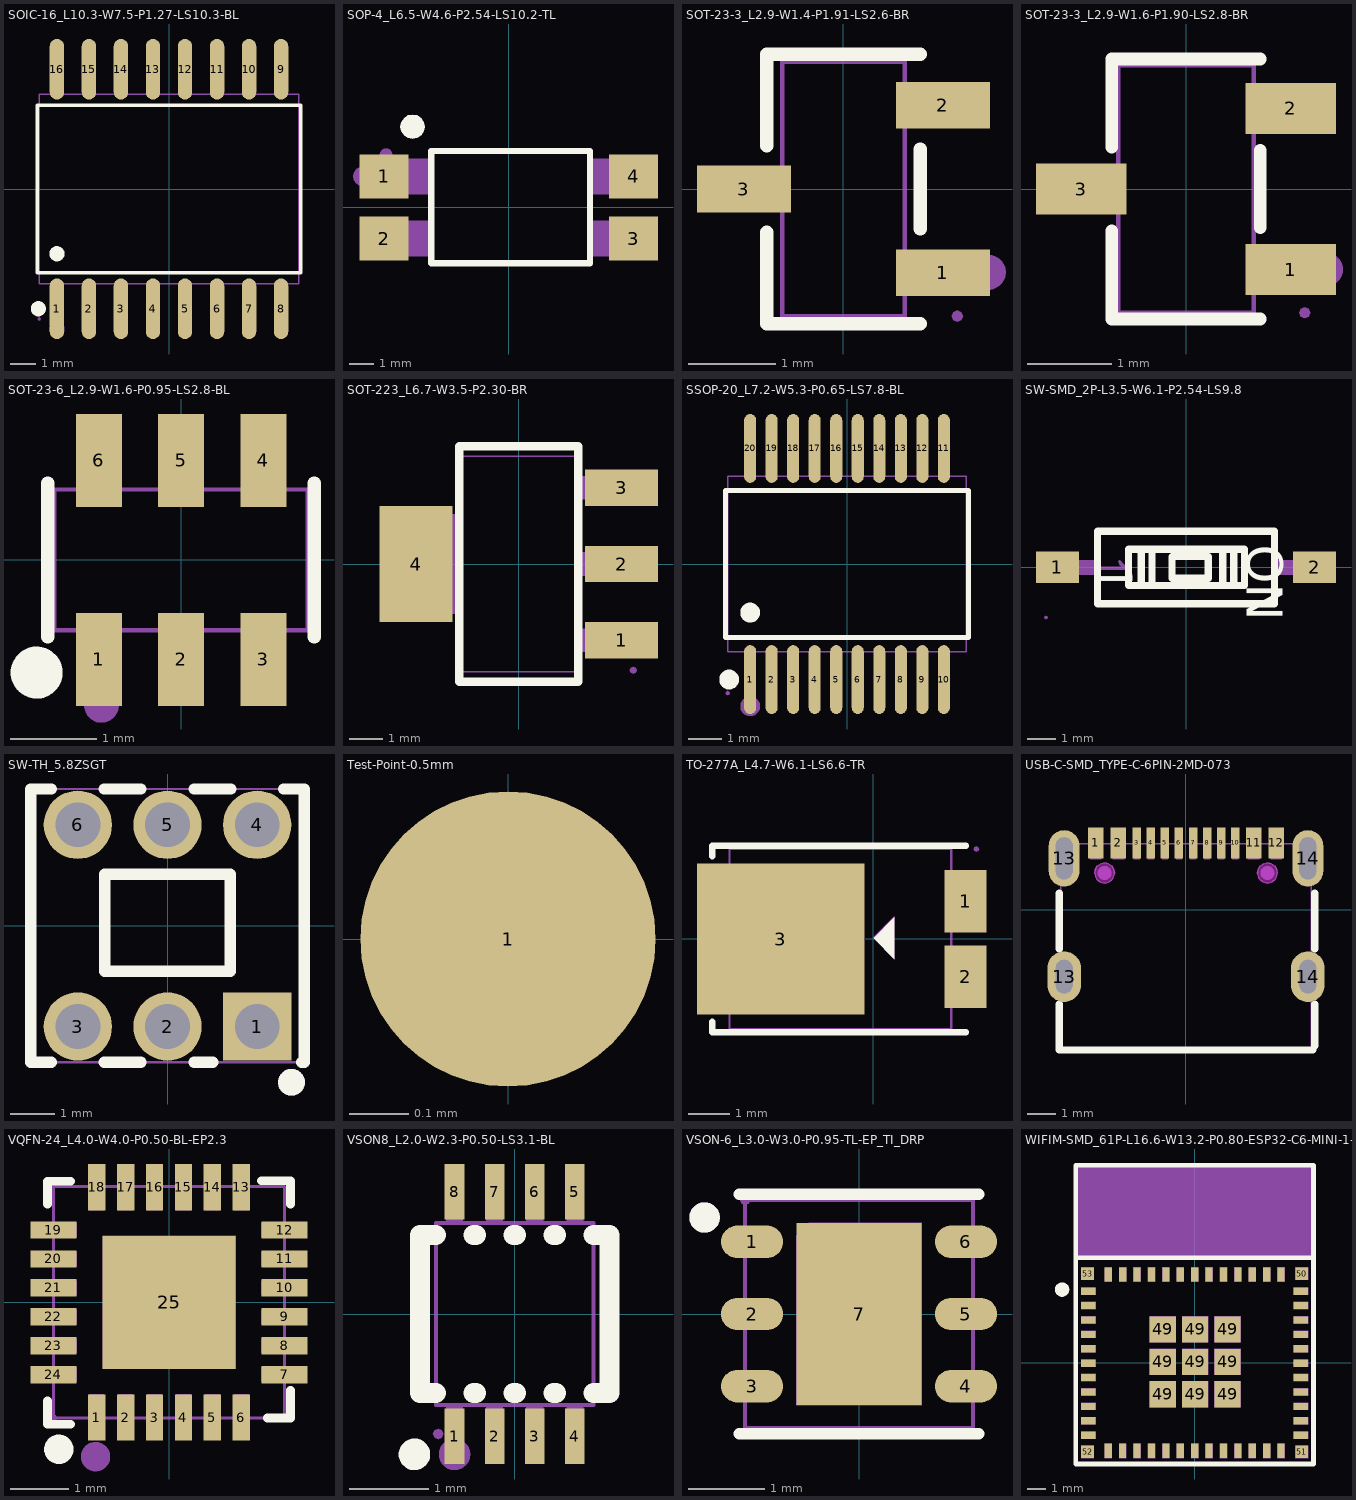
[diagram p0: the footprints below, top view; thin cyan lines are the x and y axes]
# Altium footprint library MISC84429-11.PcbLib: 64 footprints (part 4 of 4)
Each footprint in its own frame and in the unit in brackets; x right, y up, seen from the top. Pads: shape width x height; smd on the part's side, far side on the other; paste and mask are expansions set on the pad; w line width, h text height; cw(c..) or ccw(c..) is an arc to the next point about the centre after c.

## SOIC-16_L10.3-W7.5-P1.27-LS10.3-BL [mm]
pads (16):
  oval 0.574x2.401 smd: 1(-4.445,-4.75) 2(-3.175,-4.75) 3(-1.905,-4.75) 4(-0.635,-4.75) 5(0.635,-4.75) 6(1.905,-4.75) 7(3.175,-4.75) 8(4.445,-4.75) 9(4.445,4.75) 10(3.175,4.75) 11(1.905,4.75) 12(0.635,4.75) 13(-0.635,4.75) 14(-1.905,4.75) 15(-3.175,4.75) 16(-4.445,4.75)
Top Overlay:
  circle w0.3: c-5.184,-4.75 r0.15
  circle w0.3: c-4.445,-2.569 r0.15
  lines w0.152: -5.226,-3.321 5.226,-3.321 5.226,3.321 -5.226,3.321 -5.226,-3.321
Mechanical 6:
  circle w0.3: c-4.445,-5.563 r0.15
Mechanical 15:
  region: 4.24,4.338 4.24,3.74 4.65,3.74 4.65,4.338
  region: 4.24,5.162 4.24,4.327 4.65,4.327 4.65,5.162
  region: 2.97,4.338 2.97,3.74 3.38,3.74 3.38,4.338
  region: 2.97,5.162 2.97,4.327 3.38,4.327 3.38,5.162
  region: 1.7,4.338 1.7,3.74 2.11,3.74 2.11,4.338
  region: 1.7,5.162 1.7,4.327 2.11,4.327 2.11,5.162
  region: 0.43,4.338 0.43,3.74 0.84,3.74 0.84,4.338
  region: 0.43,5.162 0.43,4.327 0.84,4.327 0.84,5.162
  region: -0.84,4.338 -0.84,3.74 -0.43,3.74 -0.43,4.338
  region: -0.84,5.162 -0.84,4.327 -0.43,4.327 -0.43,5.162
  region: -2.11,4.338 -2.11,3.74 -1.7,3.74 -1.7,4.338
  region: -2.11,5.162 -2.11,4.327 -1.7,4.327 -1.7,5.162
  region: -3.38,4.338 -3.38,3.74 -2.97,3.74 -2.97,4.338
  region: -3.38,5.162 -3.38,4.327 -2.97,4.327 -2.97,5.162
  region: -4.65,4.338 -4.65,3.74 -4.24,3.74 -4.24,4.338
  region: -4.65,5.162 -4.65,4.327 -4.24,4.327 -4.24,5.162
  region: 4.24,-4.338 4.24,-3.74 4.65,-3.74 4.65,-4.338
  region: 4.24,-5.162 4.24,-4.327 4.65,-4.327 4.65,-5.162
  region: 2.97,-4.338 2.97,-3.74 3.38,-3.74 3.38,-4.338
  region: 2.97,-5.162 2.97,-4.327 3.38,-4.327 3.38,-5.162
  region: 1.7,-4.338 1.7,-3.74 2.11,-3.74 2.11,-4.338
  region: 1.7,-5.162 1.7,-4.327 2.11,-4.327 2.11,-5.162
  region: 0.43,-4.338 0.43,-3.74 0.84,-3.74 0.84,-4.338
  region: 0.43,-5.162 0.43,-4.327 0.84,-4.327 0.84,-5.162
  region: -0.84,-4.338 -0.84,-3.74 -0.43,-3.74 -0.43,-4.338
  region: -0.84,-5.162 -0.84,-4.327 -0.43,-4.327 -0.43,-5.162
  region: -2.11,-4.338 -2.11,-3.74 -1.7,-3.74 -1.7,-4.338
  region: -2.11,-5.162 -2.11,-4.327 -1.7,-4.327 -1.7,-5.162
  region: -3.38,-4.338 -3.38,-3.74 -2.97,-3.74 -2.97,-4.338
  region: -3.38,-5.162 -3.38,-4.327 -2.97,-4.327 -2.97,-5.162
  region: -4.65,-4.338 -4.65,-3.74 -4.24,-3.74 -4.24,-4.338
  region: -4.65,-5.162 -4.65,-4.327 -4.24,-4.327 -4.24,-5.162
  region: -5.085,-5.163 -5.104,-5.208 -5.15,-5.227 -5.196,-5.208 -5.215,-5.163 -5.196,-5.117 -5.15,-5.098 -5.104,-5.117
  lines w0.051: -5.15,-3.75 5.15,-3.75 5.15,3.75 -5.15,3.75 -5.15,-3.75

## SOP-4_L6.5-W4.6-P2.54-LS10.2-TL [mm]
pads (4):
  rect 2x1.8 smd: 1(-5.1,1.27) 2(-5.1,-1.27) 3(5.1,-1.27) 4(5.1,1.27)
Top Overlay:
  region: -4.433,3.302 -4.395,3.114 -4.288,2.953 -4.127,2.845 -3.937,2.807 -3.747,2.845 -3.586,2.953 -3.479,3.114 -3.441,3.303 -3.479,3.493 -3.586,3.654 -3.747,3.761 -3.937,3.799 -4.127,3.761 -4.288,3.654 -4.395,3.493 -4.433,3.305 -4.423,3.304
  lines w0.254: -3.175,-2.286 3.325,-2.286 3.325,2.314 -3.175,2.314 -3.175,-2.286
Mechanical 1:
  circle w0.4: c-5.969,1.27 r0.2
Mechanical 2:
  region: -4.764,2.163 -4.784,2.064 -4.84,1.98 -4.924,1.924 -5.023,1.904 -5.122,1.924 -5.206,1.98 -5.262,2.064 -5.282,2.163 -5.262,2.262 -5.206,2.346 -5.122,2.402 -5.023,2.422 -4.924,2.402 -4.84,2.346 -4.784,2.262
  region: -4.55,0.545 -5.15,0.545 -5.15,1.995 -4.55,1.995
  region: -3.24,0.545 -4.56,0.545 -4.56,1.995 -3.24,1.995
  region: -4.55,-1.995 -5.15,-1.995 -5.15,-0.545 -4.55,-0.545
  region: -3.24,-1.995 -4.56,-1.995 -4.56,-0.545 -3.24,-0.545
  region: 5.15,-1.995 4.55,-1.995 4.55,-0.545 5.15,-0.545
  region: 4.56,-1.995 3.24,-1.995 3.24,-0.545 4.56,-0.545
  region: 5.15,0.545 4.55,0.545 4.55,1.995 5.15,1.995
  region: 4.56,0.545 3.24,0.545 3.24,1.995 4.56,1.995
  lines w0.051: -3.25,-2.29 3.25,-2.29 3.25,2.29 -3.25,2.29 -3.25,-2.29

## SOT-23-3_L2.9-W1.4-P1.91-LS2.6-BR [mm]
pads (3):
  rect 1.07x0.532 smd: 1(1.135,-0.955) 2(1.135,0.955) 3(-1.135,0)
Top Overlay:
  lines w0.152: -0.876,-0.495 -0.876,-1.536 0.876,-1.536 ; -0.876,0.495 -0.876,1.536 0.876,1.536 ; 0.876,-0.455 0.876,0.455
Mechanical 1:
  circle w0.2: c1.651,-0.95 r0.1
Mechanical 2:
  region: 1.365,-1.45 1.346,-1.496 1.3,-1.515 1.254,-1.496 1.235,-1.45 1.254,-1.404 1.3,-1.385 1.346,-1.404
  region: -0.96,-0.212 -0.96,0.212 -0.69,0.212 -0.69,-0.212
  region: -1.3,-0.212 -1.3,0.212 -0.95,0.212 -0.95,-0.212
  region: 0.69,0.742 0.69,1.167 0.96,1.167 0.96,0.742
  region: 0.95,0.742 0.95,1.167 1.3,1.167 1.3,0.742
  region: 0.69,-1.167 0.69,-0.742 0.96,-0.742 0.96,-1.167
  region: 0.95,-1.167 0.95,-0.742 1.3,-0.742 1.3,-1.167
  lines w0.051: -0.7,-1.45 -0.7,1.45 0.7,1.45 0.7,-1.45 -0.7,-1.45

## SOT-23-3_L2.9-W1.6-P1.90-LS2.8-BR [mm]
pads (3):
  rect 1.07x0.6 smd: 1(1.235,-0.95) 2(1.235,0.95) 3(-1.235,0)
Top Overlay:
  lines w0.152: -0.876,-0.495 -0.876,-1.536 0.876,-1.536 ; -0.876,0.495 -0.876,1.536 0.876,1.536 ; 0.876,-0.455 0.876,0.455
Mechanical 1:
  circle w0.2: c1.651,-0.95 r0.1
Mechanical 2:
  region: 1.465,-1.46 1.446,-1.506 1.4,-1.525 1.354,-1.506 1.335,-1.46 1.354,-1.414 1.4,-1.395 1.446,-1.414
  region: 0.95,-1.15 0.95,-0.75 1.4,-0.75 1.4,-1.15
  region: 0.79,-1.15 0.79,-0.75 0.96,-0.75 0.96,-1.15
  region: 0.95,0.75 0.95,1.15 1.4,1.15 1.4,0.75
  region: 0.79,0.75 0.79,1.15 0.96,1.15 0.96,0.75
  region: -0.95,-0.2 -0.95,0.2 -1.4,0.2 -1.4,-0.2
  region: -0.96,-0.2 -0.96,0.2 -0.79,0.2 -0.79,-0.2
  lines w0.051: -0.8,-1.46 -0.8,1.46 0.8,1.46 0.8,-1.46 -0.8,-1.46

## SOT-23-6_L2.9-W1.6-P0.95-LS2.8-BL [mm]
pads (6):
  rect 0.532x1.072 smd: 1(-0.95,-1.149) 2(0,-1.149) 3(0.95,-1.149) 4(0.95,1.149) 5(0,1.149) 6(-0.95,1.149)
Top Overlay:
  circle w0.3: c-1.668,-1.301 r0.15
  lines w0.152: -1.539,-0.889 -1.539,0.889 ; 1.539,-0.889 1.539,0.889
Mechanical 1:
  circle w0.2: c-0.92,-1.68 r0.1
Mechanical 2:
  region: -1.398,-1.4 -1.417,-1.446 -1.463,-1.465 -1.509,-1.446 -1.528,-1.4 -1.509,-1.354 -1.463,-1.335 -1.417,-1.354
  region: -1.165,-0.925 -0.735,-0.925 -0.735,-1.4 -1.165,-1.4
  region: -1.165,-0.803 -0.735,-0.803 -0.735,-0.935 -1.165,-0.935
  region: -0.215,-0.925 0.215,-0.925 0.215,-1.4 -0.215,-1.4
  region: -0.215,-0.803 0.215,-0.803 0.215,-0.935 -0.215,-0.935
  region: 0.735,-0.925 1.165,-0.925 1.165,-1.4 0.735,-1.4
  region: 0.735,-0.803 1.165,-0.803 1.165,-0.935 0.735,-0.935
  region: 0.735,0.925 1.165,0.925 1.165,1.4 0.735,1.4
  region: 0.735,0.935 1.165,0.935 1.165,0.803 0.735,0.803
  region: -0.215,0.925 0.215,0.925 0.215,1.4 -0.215,1.4
  region: -0.215,0.935 0.215,0.935 0.215,0.803 -0.215,0.803
  region: -1.165,0.925 -0.735,0.925 -0.735,1.4 -1.165,1.4
  region: -1.165,0.935 -0.735,0.935 -0.735,0.803 -1.165,0.803
  lines w0.051: -1.463,-0.813 1.463,-0.813 1.463,0.813 -1.463,0.813 -1.463,-0.813

## SOT-223_L6.7-W3.5-P2.30-BR [mm]
pads (4):
  rect 2.2x1.1 smd: 1(3.099,-2.3) 2(3.099,0) 3(3.099,2.3)
  rect 2.2x3.5 smd: 4(-3.099,0)
Top Overlay:
  lines w0.254: -1.8,-3.55 1.8,-3.55 1.8,3.55 -1.8,3.55 -1.8,-3.55
Mechanical 1:
  circle w0.254: c3.683,-2.286 r0.127
Mechanical 2:
  region: 3.558,-3.2 3.527,-3.277 3.45,-3.308 3.373,-3.277 3.342,-3.2 3.373,-3.123 3.45,-3.092 3.527,-3.123
  region: 1.74,1.95 1.74,2.65 2.61,2.65 2.61,1.95
  region: 2.6,1.95 2.6,2.65 3.5,2.65 3.5,1.95
  region: 1.74,-0.35 1.74,0.35 2.61,0.35 2.61,-0.35
  region: 2.6,-0.35 2.6,0.35 3.5,0.35 3.5,-0.35
  region: 1.74,-2.65 1.74,-1.95 2.61,-1.95 2.61,-2.65
  region: 2.6,-2.65 2.6,-1.95 3.5,-1.95 3.5,-2.65
  region: -2.61,-1.5 -2.61,1.5 -1.74,1.5 -1.74,-1.5
  region: -3.5,-1.5 -3.5,1.5 -2.6,1.5 -2.6,-1.5
  lines w0.051: -1.75,-3.25 -1.75,3.25 1.75,3.25 1.75,-3.25 -1.75,-3.25

## SSOP-20_L7.2-W5.3-P0.65-LS7.8-BL [mm]
pads (20):
  oval 0.364x2.082 smd: 1(-2.925,-3.491) 2(-2.275,-3.491) 3(-1.625,-3.491) 4(-0.975,-3.491) 5(-0.325,-3.491) 6(0.325,-3.491) 7(0.975,-3.491) 8(1.625,-3.491) 9(2.275,-3.491) 10(2.925,-3.491) 11(2.925,3.491) 12(2.275,3.491) 13(1.625,3.491) 14(0.975,3.491) 15(0.325,3.491) 16(-0.325,3.491) 17(-0.975,3.491) 18(-1.625,3.491) 19(-2.275,3.491) 20(-2.925,3.491)
Top Overlay:
  circle w0.3: c-2.925,-1.469 r0.15
  circle w0.3: c-3.559,-3.491 r0.15
  lines w0.152: -3.676,-2.221 -3.676,2.221 3.676,2.221 3.676,-2.221 -3.676,-2.221
Mechanical 1:
  circle w0.3: c-2.925,-4.3 r0.15
Mechanical 2:
  drawing of 45 lines, arcs and shapes, not listed

## SW-SMD_2P-L3.5-W6.1-P2.54-LS9.8 [mm]
pads (2):
  rect 1.5x1.1 smd: 1(-4.5,0) 2(4.5,0)
Top Overlay:
  lines w0.254: -1.57,-0.635 -1.57,0.635 ; -1.189,-0.635 -1.189,0.635 ; 1.288,-0.635 1.288,0.635 ; 1.669,-0.635 1.669,0.635 ; -3.1,-1.27 -3.1,1.27 3.1,1.27 3.1,-1.27 -3.1,-1.27 ; -2.014,-0.635 2.05,-0.635 2.05,0.635 -2.014,0.635 -2.014,-0.635 ; -0.49,-0.381 0.78,-0.381 0.78,0.381 -0.49,0.381 -0.49,-0.381
  text "ON" at 2.134,0.787 h1.27
  text "1" at -3.13,0.19 h1.27
Mechanical 1:
  region: -2.315,0.26 -2.335,0.26 -2.375,0.22 -2.355,0.15 -2.315,0.08 -2.255,0.02 -3.075,0.02 -3.085,0.03 -3.105,0.03 -3.135,0 -3.135,-0.04 -3.125,-0.07 -3.095,-0.08 -2.105,-0.08 -2.09,-0.075 -2.08,-0.065 -2.07,-0.055 -2.065,-0.03 -2.075,-0.01 -2.095,0.02 -2.215,0.14 -2.275,0.24
Mechanical 2:
  region: -4.835,-1.75 -4.854,-1.796 -4.9,-1.815 -4.946,-1.796 -4.965,-1.75 -4.946,-1.704 -4.9,-1.685 -4.854,-1.704
  region: 3.09,-0.25 3.09,0.25 4.41,0.25 4.41,-0.25
  region: 4.4,-0.25 4.4,0.25 4.9,0.25 4.9,-0.25
  region: -4.41,-0.25 -4.41,0.25 -3.09,0.25 -3.09,-0.25
  region: -4.9,-0.25 -4.9,0.25 -4.4,0.25 -4.4,-0.25
  lines w0.051: -3.1,-1.27 -3.1,1.27 3.1,1.27 3.1,-1.27 -3.1,-1.27

## SW-TH_5.8ZSGT [mm]
pads (6):
  rect 1.524x1.524 hole 1: 1(2,-2.25)
  round 1.524 hole 1: 2(0,-2.25) 3(-2,-2.25) 4(2,2.25) 5(0,2.25) 6(-2,2.25)
Top Overlay:
  circle w0.3: c2.766,-3.493 r0.15
  lines w0.254: -2.591,-3.047 -3.048,-3.047 -3.048,3.047 -2.591,3.047 ; -1.409,-3.047 -0.591,-3.047 ; -1.409,3.047 -0.591,3.047 ; 0.591,-3.047 1.01,-3.047 ; 0.591,3.047 1.409,3.047 ; 2.591,3.047 3.048,3.047 ; 2.99,-3.047 3.048,-3.047 3.048,3.048 ; -1.397,-1.016 1.397,-1.016 1.397,1.143 -1.397,1.143 -1.397,-1.016
Mechanical 1:
  circle w0.3: c2.766,-3.493 r0.15
Mechanical 2:
  region: 3.113,-3.048 3.094,-3.094 3.048,-3.113 3.002,-3.094 2.983,-3.048 3.002,-3.002 3.048,-2.983 3.094,-3.002
  region: 2.408,2.25 2.377,2.094 2.288,1.962 2.156,1.873 2,1.842 1.844,1.873 1.712,1.962 1.623,2.094 1.592,2.25 1.623,2.406 1.712,2.538 1.844,2.627 2,2.658 2.156,2.627 2.288,2.538 2.377,2.406
  region: 0.408,2.25 0.377,2.094 0.288,1.962 0.156,1.873 0,1.842 -0.156,1.873 -0.288,1.962 -0.377,2.094 -0.408,2.25 -0.377,2.406 -0.288,2.538 -0.156,2.627 0,2.658 0.156,2.627 0.288,2.538 0.377,2.406
  region: -1.592,2.25 -1.623,2.094 -1.712,1.962 -1.844,1.873 -2,1.842 -2.156,1.873 -2.288,1.962 -2.377,2.094 -2.408,2.25 -2.377,2.406 -2.288,2.538 -2.156,2.627 -2,2.658 -1.844,2.627 -1.712,2.538 -1.623,2.406
  region: -1.592,-2.25 -1.623,-2.406 -1.712,-2.538 -1.844,-2.627 -2,-2.658 -2.156,-2.627 -2.288,-2.538 -2.377,-2.406 -2.408,-2.25 -2.377,-2.094 -2.288,-1.962 -2.156,-1.873 -2,-1.842 -1.844,-1.873 -1.712,-1.962 -1.623,-2.094
  region: 0.408,-2.25 0.377,-2.406 0.288,-2.538 0.156,-2.627 0,-2.658 -0.156,-2.627 -0.288,-2.538 -0.377,-2.406 -0.408,-2.25 -0.377,-2.094 -0.288,-1.962 -0.156,-1.873 0,-1.842 0.156,-1.873 0.288,-1.962 0.377,-2.094
  region: 2.408,-2.25 2.377,-2.406 2.288,-2.538 2.156,-2.627 2,-2.658 1.844,-2.627 1.712,-2.538 1.623,-2.406 1.592,-2.25 1.623,-2.094 1.712,-1.962 1.844,-1.873 2,-1.842 2.156,-1.873 2.288,-1.962 2.377,-2.094
  lines w0.051: -3.048,-3.048 3.048,-3.048 3.048,3.048 -3.048,3.048 -3.048,-3.048

## Test-Point-0.5mm [mm]
pads (1):
  round 0.5 smd: 1(0,0)

## TO-277A_L4.7-W6.1-LS6.6-TR [mm]
pads (3):
  rect 1x1.5 smd: 1(2.21,0.9) 2(2.21,-0.9)
  rect 4x3.6 smd: 3(-2.21,0)
Top Overlay:
  region: 0.01,0.02 0.51,0.52 0.51,-0.48
  lines w0.152: -3.844,-1.98 -3.844,-2.229 2.218,-2.229 ; -3.844,1.98 -3.844,2.229 2.218,2.229
Mechanical 1:
  region: 0,0.04 0.5,0.54 0.5,-0.46
Mechanical 2:
  region: 2.53,2.15 2.511,2.104 2.465,2.085 2.419,2.104 2.4,2.15 2.419,2.196 2.465,2.215 2.511,2.196
  region: -4.033,0.9 -3.538,0.9 -3.538,1.54 -0.238,1.54 -0.238,-1.52 -3.538,-1.52 -3.538,-0.9 -4.033,-0.899 -4.032,0
  region: 1.863,1.351 2.465,1.35 2.465,0.45 1.862,0.45 1.862,0.897
  region: 1.863,-0.451 2.465,-0.45 2.465,-1.35 1.862,-1.349 1.862,-0.913
  lines w0.051: -3.432,-2.15 -3.432,2.15 1.868,2.15 1.868,-2.15 -3.432,-2.15

## USB-C-SMD_TYPE-C-6PIN-2MD-073 [mm]
pads (16):
  rect 0.55x1.1 smd paste-100 mask+0.05: 1(-3.2,2.375) 2(-2.4,2.375) 11(2.4,2.375) 12(3.2,2.375)
  rect 0.3x1.1 smd paste-100 mask+0.05: 3(-1.75,2.375) 4(-1.25,2.375) 5(-0.75,2.375) 6(-0.25,2.375) 7(0.25,2.375) 8(0.75,2.375) 9(1.25,2.375) 10(1.75,2.375)
  oval 1.2x1.8 hole 0.6 slot 1.2 at 90 deg paste+0 mask-0.25: 13(-4.325,-2.375) 14(4.325,-2.375)
  oval 1.1x2 hole 0.6 slot 1.5 at 90 deg paste+0 mask-0.2: 13(-4.325,1.825) 14(4.325,1.825)
Top Overlay:
  lines w0.254: -4.5,-3.356 -4.5,-4.975 4.5,-4.975 ; -4.5,-1.394 -4.5,0.594 ; 4.572,-4.826 4.572,-3.353 ; 4.572,-1.397 4.572,0.597
Top Paste:
  drawing of 16 lines, arcs and shapes, not listed
Keep-Out Layer:
  circle w0.013: c-2.89,1.305 r0.35
  circle w0.013: c-2.89,1.305 r0.35
  circle w0.013: c2.89,1.305 r0.35
  circle w0.013: c2.89,1.305 r0.35
  board cut-out: -2.533,1.305 -2.56,1.168 -2.638,1.053 -2.753,0.975 -2.89,0.948 -3.026,0.975 -3.142,1.053 -3.22,1.168 -3.247,1.305 -3.22,1.441 -3.142,1.557 -3.026,1.635 -2.89,1.662 -2.753,1.635 -2.638,1.557 -2.56,1.441
  board cut-out: 3.247,1.305 3.22,1.168 3.142,1.053 3.027,0.975 2.89,0.948 2.754,0.975 2.638,1.053 2.56,1.168 2.533,1.305 2.56,1.441 2.638,1.557 2.754,1.635 2.89,1.662 3.027,1.635 3.142,1.557 3.22,1.441
  region: -2.533,1.305 -2.56,1.168 -2.638,1.053 -2.753,0.975 -2.89,0.948 -3.026,0.975 -3.142,1.053 -3.22,1.168 -3.247,1.305 -3.22,1.441 -3.142,1.557 -3.026,1.635 -2.89,1.662 -2.753,1.635 -2.638,1.557 -2.56,1.441
  region: 3.247,1.305 3.22,1.168 3.142,1.053 3.027,0.975 2.89,0.948 2.754,0.975 2.638,1.053 2.56,1.168 2.533,1.305 2.56,1.441 2.638,1.557 2.754,1.635 2.89,1.662 3.027,1.635 3.142,1.557 3.22,1.441
  region: -2.533,1.305 -2.56,1.168 -2.638,1.053 -2.753,0.975 -2.89,0.948 -3.026,0.975 -3.142,1.053 -3.22,1.168 -3.247,1.305 -3.22,1.441 -3.142,1.557 -3.026,1.635 -2.89,1.662 -2.753,1.635 -2.638,1.557 -2.56,1.441
  region: 3.247,1.305 3.22,1.168 3.142,1.053 3.027,0.975 2.89,0.948 2.754,0.975 2.638,1.053 2.56,1.168 2.533,1.305 2.56,1.441 2.638,1.557 2.754,1.635 2.89,1.662 3.027,1.635 3.142,1.557 3.22,1.441
  lines w0.005: -3.247,1.305 -3.22,1.441 -3.142,1.557 -3.026,1.635 -2.89,1.662 -2.753,1.635 -2.638,1.557 -2.56,1.441 -2.533,1.305 -2.56,1.168 -2.638,1.053 -2.753,0.975 -2.89,0.948 -3.026,0.975 -3.142,1.053 -3.22,1.168 -3.247,1.305 ; 2.533,1.305 2.56,1.441 2.638,1.557 2.754,1.635 2.89,1.662 3.027,1.635 3.142,1.557 3.22,1.441 3.247,1.305 3.22,1.168 3.142,1.053 3.027,0.975 2.89,0.948 2.754,0.975 2.638,1.053 2.56,1.168 2.533,1.305
Mechanical 1:
  circle w0.013: c-2.89,1.305 r0.35
  circle w0.013: c2.89,1.305 r0.35
  circle w0.25: c-2.89,1.305 r0.125
  circle w0.25: c2.89,1.305 r0.125
  lines w0.005: -3.247,1.305 -3.22,1.441 -3.142,1.557 -3.026,1.635 -2.89,1.662 -2.753,1.635 -2.638,1.557 -2.56,1.441 -2.533,1.305 -2.56,1.168 -2.638,1.053 -2.753,0.975 -2.89,0.948 -3.026,0.975 -3.142,1.053 -3.22,1.168 -3.247,1.305 ; 2.533,1.305 2.56,1.441 2.638,1.557 2.754,1.635 2.89,1.662 3.027,1.635 3.142,1.557 3.22,1.441 3.247,1.305 3.22,1.168 3.142,1.053 3.027,0.975 2.89,0.948 2.754,0.975 2.638,1.053 2.56,1.168 2.533,1.305
Mechanical 2:
  region: -4.385,2.649 -4.404,2.603 -4.45,2.584 -4.496,2.603 -4.515,2.649 -4.496,2.695 -4.45,2.714 -4.404,2.695
  region: -1.85,2.649 -1.65,2.649 -1.65,1.799 -1.85,1.799
  region: -0.85,2.649 -0.65,2.649 -0.65,1.799 -0.85,1.799
  region: -1.35,2.649 -1.15,2.649 -1.15,1.799 -1.35,1.799
  region: -0.35,2.649 -0.15,2.649 -0.15,1.799 -0.35,1.799
  region: 0.15,2.649 0.35,2.649 0.35,1.799 0.15,1.799
  region: 0.65,2.649 0.85,2.649 0.85,1.799 0.65,1.799
  region: 1.15,2.649 1.35,2.649 1.35,1.799 1.15,1.799
  region: 1.65,2.649 1.85,2.649 1.85,1.799 1.65,1.799
  region: -3.4,2.649 -3,2.649 -3,1.799 -3.4,1.799
  region: -2.6,2.649 -2.2,2.649 -2.2,1.799 -2.6,1.799
  region: 2.2,2.649 2.6,2.649 2.6,1.799 2.2,1.799
  region: 3,2.649 3.4,2.649 3.4,1.799 3,1.799
  region: -4.45,2.349 -4.2,2.349 -4.2,1.249 -4.45,1.249
  region: 4.2,2.349 4.45,2.349 4.45,1.249 4.2,1.249
  region: -4.45,-2.025 -4.2,-2.025 -4.2,-2.725 -4.45,-2.725
  region: 4.2,-2.025 4.45,-2.025 4.45,-2.725 4.2,-2.725
  lines w0.051: -4.45,-5.001 -4.45,2.349 4.45,2.349 4.45,-5.001 -4.45,-5.001

## VQFN-24_L4.0-W4.0-P0.50-BL-EP2.3 [mm]
pads (25):
  rect 0.3x0.8 smd paste-100 mask+0.051: 1(-1.25,-1.992) 2(-0.75,-1.991) 3(-0.25,-1.991) 4(0.25,-1.991) 5(0.75,-1.991) 6(1.25,-1.991) 13(1.25,1.992) 14(0.75,1.992) 15(0.25,1.992) 16(-0.25,1.992) 17(-0.75,1.992) 18(-1.25,1.992)
  rect 0.8x0.3 smd paste-100 mask+0.051: 7(1.998,-1.25) 8(1.998,-0.75) 9(1.998,-0.25) 10(1.998,0.25) 11(1.998,0.75) 12(1.998,1.25) 19(-1.998,1.25) 20(-1.998,0.75) 21(-1.998,0.25) 22(-1.998,-0.25) 23(-1.998,-0.75) 24(-1.998,-1.25)
  rect 2.3x2.3 smd paste-100 mask+0.051: 25(0.001,-0.001)
Top Overlay:
  circle w0.254: c-1.905,-2.54 r0.127
  lines w0.15: -2.1,1.696 -2.1,2.096 -1.7,2.096 ; -2.1,-1.7 -2.1,-2.104 -1.7,-2.104 ; 1.6,2.1 2.1,2.1 2.1,1.7 ; 1.7,-2 2.1,-2 2.1,-1.524
Top Paste:
  region: 1.4,1.592 1.4,2.392 1.1,2.392 1.1,1.592
  region: -1.4,2.392 -1.4,1.592 -1.1,1.592 -1.1,2.392
  region: 0.9,1.592 0.9,2.392 0.6,2.392 0.6,1.592
  region: 0.4,1.592 0.4,2.392 0.1,2.392 0.1,1.592
  region: -0.1,1.592 -0.1,2.392 -0.4,2.392 -0.4,1.592
  region: -0.9,2.392 -0.9,1.592 -0.6,1.592 -0.6,2.392
  region: 2.398,1.1 2.398,1.4 1.598,1.4 1.598,1.1
  region: -2.398,1.4 -2.398,1.1 -1.598,1.1 -1.598,1.4
  region: 0.95,-0.95 0.95,0.95 -0.95,0.95 -0.95,-0.95
  region: 1.598,0.9 1.598,0.6 2.398,0.6 2.398,0.9
  region: -2.398,0.9 -2.398,0.6 -1.598,0.6 -1.598,0.9
  region: -2.398,0.4 -2.398,0.1 -1.598,0.1 -1.598,0.4
  region: 1.598,0.4 1.598,0.1 2.398,0.1 2.398,0.4
  region: -2.398,-0.1 -2.398,-0.4 -1.598,-0.4 -1.598,-0.1
  region: 1.598,-0.1 1.598,-0.4 2.398,-0.4 2.398,-0.1
  region: -2.398,-0.6 -2.398,-0.9 -1.598,-0.9 -1.598,-0.6
  region: 1.598,-0.6 1.598,-0.9 2.398,-0.9 2.398,-0.6
  region: -2.398,-1.1 -2.398,-1.4 -1.598,-1.4 -1.598,-1.1
  region: 1.598,-1.1 1.598,-1.4 2.398,-1.4 2.398,-1.1
  region: 1.4,-2.391 1.4,-1.591 1.1,-1.591 1.1,-2.391
  region: 0.9,-2.391 0.9,-1.591 0.6,-1.591 0.6,-2.391
  region: -0.4,-1.591 -0.4,-2.391 -0.1,-2.391 -0.1,-1.591
  region: 0.4,-2.391 0.4,-1.591 0.1,-1.591 0.1,-2.391
  region: -0.9,-1.591 -0.9,-2.391 -0.6,-2.391 -0.6,-1.591
  region: -1.1,-2.392 -1.1,-1.592 -1.4,-1.592 -1.4,-2.392
Mechanical 1:
  circle w0.254: c-1.27,-2.667 r0.127
Mechanical 2:
  region: -1.935,-2 -1.954,-2.046 -2,-2.065 -2.046,-2.046 -2.065,-2 -2.046,-1.954 -2,-1.935 -1.954,-1.954
  region: -1.125,-1.992 -1.375,-1.992 -1.375,-1.592 -1.125,-1.592
  region: -0.625,-1.992 -0.875,-1.992 -0.875,-1.592 -0.625,-1.592
  region: -0.125,-1.992 -0.375,-1.992 -0.375,-1.592 -0.125,-1.592
  region: 0.375,-1.992 0.125,-1.992 0.125,-1.592 0.375,-1.592
  region: 0.875,-1.992 0.625,-1.992 0.625,-1.592 0.875,-1.592
  region: 1.375,-1.992 1.125,-1.992 1.125,-1.592 1.375,-1.592
  region: 1.598,-1.375 1.598,-1.125 1.998,-1.125 1.998,-1.375
  region: 1.598,-0.875 1.598,-0.625 1.998,-0.625 1.998,-0.875
  region: 1.598,-0.375 1.598,-0.125 1.998,-0.125 1.998,-0.375
  region: 1.598,0.125 1.598,0.375 1.998,0.375 1.998,0.125
  region: 1.598,0.625 1.598,0.875 1.998,0.875 1.998,0.625
  region: 1.598,1.125 1.598,1.375 1.998,1.375 1.998,1.125
  region: 1.125,1.992 1.375,1.992 1.375,1.592 1.125,1.592
  region: 0.625,1.992 0.875,1.992 0.875,1.592 0.625,1.592
  region: 0.125,1.992 0.375,1.992 0.375,1.592 0.125,1.592
  region: -0.375,1.992 -0.125,1.992 -0.125,1.592 -0.375,1.592
  region: -0.875,1.992 -0.625,1.992 -0.625,1.592 -0.875,1.592
  region: -1.375,1.992 -1.125,1.992 -1.125,1.592 -1.375,1.592
  region: -1.598,1.375 -1.598,1.125 -1.998,1.125 -1.998,1.375
  region: -1.598,0.875 -1.598,0.625 -1.998,0.625 -1.998,0.875
  region: -1.598,0.375 -1.598,0.125 -1.998,0.125 -1.998,0.375
  region: -1.598,-0.125 -1.598,-0.375 -1.998,-0.375 -1.998,-0.125
  region: -1.598,-0.625 -1.598,-0.875 -1.998,-0.875 -1.998,-0.625
  region: -1.598,-1.125 -1.598,-1.375 -1.998,-1.375 -1.998,-1.125
  region: -1.149,-1.151 -1.149,1.149 1.151,1.149 1.151,-1.151
  lines w0.051: -2,-2 2,-2 2,2 -2,2 -2,-2

## VSON8_L2.0-W2.3-P0.50-LS3.1-BL [mm]
pads (8):
  rect 0.25x0.7 smd: 1(-0.762,-1.55) 2(-0.254,-1.55) 3(0.254,-1.55) 4(0.762,-1.55) 5(0.762,1.55) 6(0.254,1.55) 7(-0.254,1.55) 8(-0.762,1.55)
Top Overlay:
  circle w0.2: c-1.27,-1.778 r0.1
  lines w0.254: -1,-1 -1.2,-1 -1.2,1 -1,1 ; -0.524,-1 -0.492,-1 ; -0.524,1 -0.492,1 ; -0.016,-1 0.016,-1 ; -0.016,1 0.016,1 ; 0.492,-1 0.524,-1 ; 0.492,1 0.524,1 ; 1,-1 1.2,-1 1.2,1 1,1
Mechanical 1:
  circle w0.2: c-0.762,-1.778 r0.1
Mechanical 2:
  region: -0.905,-1.52 -0.924,-1.566 -0.97,-1.585 -1.016,-1.566 -1.035,-1.52 -1.016,-1.474 -0.97,-1.455 -0.924,-1.474
  region: -0.867,1.14 -0.867,1.285 -0.657,1.285 -0.657,1.14
  region: -0.867,1.275 -0.867,1.55 -0.657,1.55 -0.657,1.275
  region: -0.359,1.14 -0.359,1.285 -0.149,1.285 -0.149,1.14
  region: -0.359,1.275 -0.359,1.55 -0.149,1.55 -0.149,1.275
  region: 0.149,1.14 0.149,1.285 0.359,1.285 0.359,1.14
  region: 0.149,1.275 0.149,1.55 0.359,1.55 0.359,1.275
  region: 0.657,1.14 0.657,1.285 0.867,1.285 0.867,1.14
  region: 0.657,1.275 0.657,1.55 0.867,1.55 0.867,1.275
  region: 0.657,-1.285 0.657,-1.14 0.867,-1.14 0.867,-1.285
  region: 0.657,-1.55 0.657,-1.275 0.867,-1.275 0.867,-1.55
  region: 0.149,-1.285 0.149,-1.14 0.359,-1.14 0.359,-1.285
  region: 0.149,-1.55 0.149,-1.275 0.359,-1.275 0.359,-1.55
  region: -0.359,-1.285 -0.359,-1.14 -0.149,-1.14 -0.149,-1.285
  region: -0.359,-1.55 -0.359,-1.275 -0.149,-1.275 -0.149,-1.55
  region: -0.867,-1.285 -0.867,-1.14 -0.657,-1.14 -0.657,-1.285
  region: -0.867,-1.55 -0.867,-1.275 -0.657,-1.275 -0.657,-1.55
  lines w0.051: -1,-1.15 1,-1.15 1,1.15 -1,1.15 -1,-1.15

## VSON-6_L3.0-W3.0-P0.95-TL-EP_TI_DRP [mm]
pads (7):
  oval 0.817x0.427 smd: 1(-1.407,0.95) 2(-1.407,0) 3(-1.407,-0.95) 4(1.407,-0.95) 5(1.407,0) 6(1.407,0.95)
  rect 1.65x2.4 smd: 7(0,0)
Top Overlay:
  circle w0.2: c-2.032,1.27 r0.1
  lines w0.152: -1.576,-1.576 1.576,-1.576 ; -1.576,1.576 1.576,1.576
Mechanical 6:
  circle w0.2: c-2.032,1.27 r0.1
Mechanical 15:
  region: -0.66,1.2 0.825,1.2 0.825,-1.2 -0.825,-1.2 -0.825,1.035
  region: 1.5,0.797 1.1,0.797 1.1,1.102 1.5,1.102
  region: 1.5,-0.152 1.1,-0.152 1.1,0.152 1.5,0.152
  region: 1.5,-1.102 1.1,-1.102 1.1,-0.797 1.5,-0.797
  region: -1.5,-1.102 -1.1,-1.102 -1.1,-0.797 -1.5,-0.797
  region: -1.5,-0.152 -1.1,-0.152 -1.1,0.152 -1.5,0.152
  region: -1.5,0.797 -1.1,0.797 -1.1,1.102 -1.5,1.102
  region: -1.435,1.5 -1.454,1.454 -1.5,1.435 -1.546,1.454 -1.565,1.5 -1.546,1.546 -1.5,1.565 -1.454,1.546
  lines w0.051: -1.5,-1.5 -1.5,1.5 1.5,1.5 1.5,-1.5 -1.5,-1.5

## WIFIM-SMD_61P-L16.6-W13.2-P0.80-ESP32-C6-MINI-1-N4 [mm]
pads (61):
  rect 0.8x0.4 smd paste+0 mask+0.05: 1(-5.9,3.975) 2(-5.9,3.175) 3(-5.9,2.375) 4(-5.9,1.575) 5(-5.9,0.775) 6(-5.9,-0.025) 7(-5.9,-0.825) 8(-5.9,-1.625) 9(-5.9,-2.425) 10(-5.9,-3.225) 11(-5.9,-4.025) 25(5.9,-4.025) 26(5.9,-3.225) 27(5.9,-2.425) 28(5.9,-1.625) 29(5.9,-0.825) 30(5.9,-0.025) 31(5.9,0.775) 32(5.9,1.575) 33(5.9,2.375) 34(5.9,3.175) 35(5.9,3.975)
  rect 0.4x0.8 smd paste+0 mask+0.05: 12(-4.8,-4.9) 13(-4,-4.9) 14(-3.2,-4.9) 15(-2.4,-4.9) 16(-1.6,-4.9) 17(-0.8,-4.9) 18(0,-4.9) 19(0.8,-4.9) 20(1.6,-4.9) 21(2.4,-4.9) 22(3.2,-4.9) 23(4,-4.9) 24(4.8,-4.9) 36(4.8,4.9) 37(4,4.9) 38(3.2,4.9) 39(2.4,4.9) 40(1.6,4.9) 41(0.8,4.9) 42(0,4.9) 43(-0.8,4.9) 44(-1.6,4.9) 45(-2.4,4.9) 46(-3.2,4.9) 47(-4,4.9) 48(-4.8,4.9)
  rect 1.45x1.45 smd paste+0 mask+0.05: 49(-1.775,-1.75) 49(-1.775,0.05) 49(-1.775,1.85) 49(0.025,-1.75) 49(0.025,0.05) 49(0.025,1.85) 49(1.825,-1.75) 49(1.825,0.05) 49(1.825,1.85)
  rect 0.7x0.7 smd paste+0 mask+0.05: 50(5.95,4.95) 51(5.95,-4.95) 52(-5.95,-4.95) 53(-5.95,4.95)
Top Overlay:
  circle w0.4: c-7.366,4.064 r0.2
  lines w0.254: -6.604,5.842 6.604,5.842 ; -6.6,-5.625 6.6,-5.625 6.6,10.975 -6.6,10.975 -6.6,-5.625
Mechanical 1:
  region: -6.604,10.922 -6.604,5.842 6.604,5.842 6.604,10.922
Mechanical 2:
  drawing of 66 lines, arcs and shapes, not listed